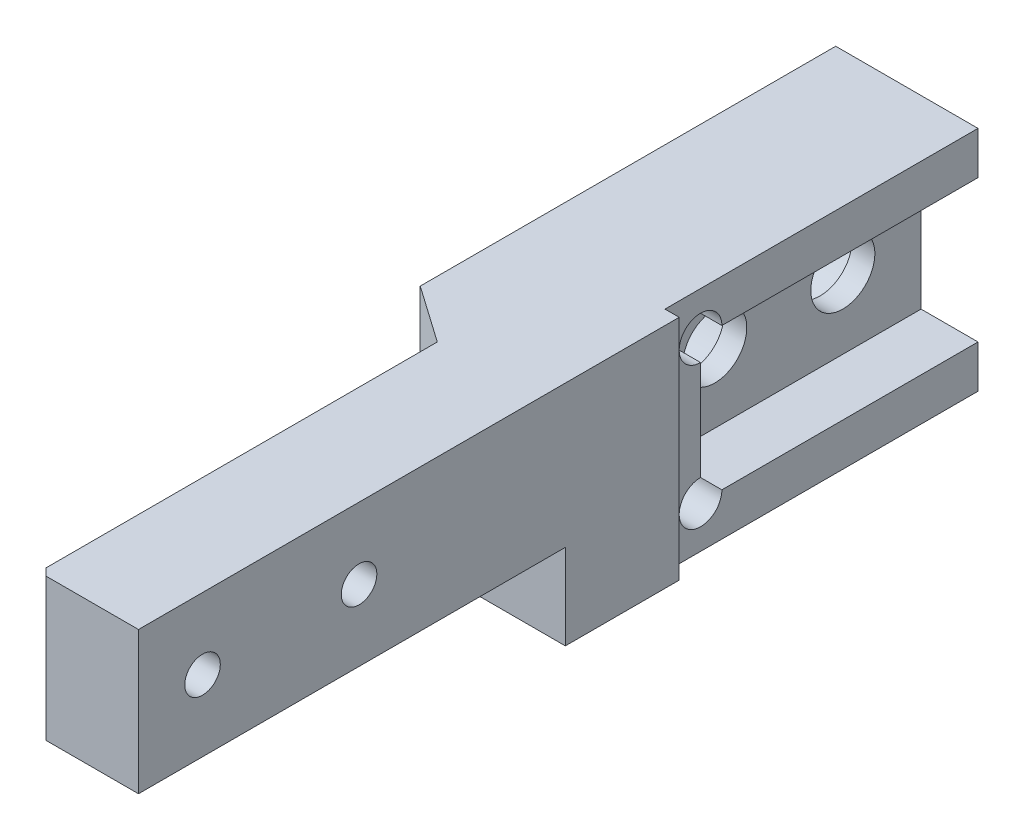
from build123d import *

# Parameters (mm, degrees)
SKETCH_1_W                   = 20
SKETCH_1_H                   = 60
EXTRUDE_1_DEPTH              = 8
SKETCH_2_W                   = 19.5
SKETCH_2_H                   = 10
CUT_EXTRUDE_1_DEPTH          = 14
CHAMFER_1_SIZE               = 3
CUT_EXTRUDE_3_DEPTH          = 36.440090293
CUT_EXTRUDE_3_DEPTH_BACK     = 36.440090293
CHAMFER_2_SIZE               = 0.5
SKETCH_6_R                   = 1.5
CUT_EXTRUDE_4_DEPTH          = 14
HOLE_WIZARD_M4_1_D           = 4.5
HOLE_WIZARD_M4_1_CBORE_D     = 8
HOLE_WIZARD_M4_1_CBORE_DEPTH = 4.4
SKETCH_11_W                  = 10
SKETCH_11_H                  = 22
CUT_EXTRUDE_7_DEPTH          = 36.440090293
SKETCH_12_W                  = 30
SKETCH_12_H                  = 6
CUT_EXTRUDE_8_DEPTH          = 37.932370625
CUT_EXTRUDE_9_DEPTH          = 34.166247904
FILLET_2_R                   = 3
SKETCH_14_W                  = 18.511605667
SKETCH_14_H                  = 56.283608206
CUT_EXTRUDE_10_DEPTH         = 36.440090293
HOLE_WIZARD_M3_1_D           = 2.5


with BuildPart() as part:
    # 草图1 → 凸台-拉伸1 (new, symmetric)
    with BuildSketch(Plane(origin=(0, 0, 0), x_dir=(1, 0, 0), z_dir=(0, 1, 0))):
        Rectangle(SKETCH_1_W, SKETCH_1_H)
    extrude(amount=EXTRUDE_1_DEPTH, both=True)

    # 草图2 → 切除-拉伸1 (cut)
    with BuildSketch(Plane(origin=(10, 0, 0), x_dir=(0, 0, -1), z_dir=(1, 0, 0))):
        with Locations((20.25, 0)):
            Rectangle(SKETCH_2_W, SKETCH_2_H)
    extrude(amount=-CUT_EXTRUDE_1_DEPTH, mode=Mode.SUBTRACT)

    # 倒角1
    chamfer_1_edges = [part.edges().sort_by_distance(p)[0] for p in [
        (10, -6.5, -30),
        (10, 6.5, -30),
    ]]
    chamfer(chamfer_1_edges, length=CHAMFER_1_SIZE)

    # 草图5 → 切除-拉伸3 (cut, two sides: drawn at the far end of the back side and taken through both)
    with BuildSketch(Plane.XZ.offset(8).offset(-CUT_EXTRUDE_3_DEPTH_BACK)):
        Polygon((-6, 164.19339757), (-6, 30), (-6, 2), (-10, -0.800830153), (-119.92479595, -77.771000913), (-362.743295595, 36.555933952), (-248.818499645, 278.520332435), align=None)
    extrude(amount=CUT_EXTRUDE_3_DEPTH + CUT_EXTRUDE_3_DEPTH_BACK, mode=Mode.SUBTRACT)

    # 倒角2
    chamfer_2_edges = [part.edges().sort_by_distance(p)[0] for p in [
        (-6, 0, 30),
        (10, 0, 30),
    ]]
    chamfer(chamfer_2_edges, length=CHAMFER_2_SIZE)

    # 草图6 → 切除-拉伸4 (cut)
    with BuildSketch(Plane(origin=(10, 0, 0), x_dir=(0, 0, -1), z_dir=(1, 0, 0))):
        with Locations((10.5, 5)):
            Circle(SKETCH_6_R)
        with Locations((10.5, -5)):
            Circle(SKETCH_6_R)
    extrude(amount=-CUT_EXTRUDE_4_DEPTH, mode=Mode.SUBTRACT)

    # M4 六角凹头螺钉的柱形沉头孔1 (through all)
    with Locations(Plane.ZY.offset(10)):
        with Locations((-15.500000304, 6.53e-07), (-24.500000304, 6.53e-07)):
            CounterBoreHole(HOLE_WIZARD_M4_1_D / 2, HOLE_WIZARD_M4_1_CBORE_D / 2, HOLE_WIZARD_M4_1_CBORE_DEPTH)

    # 草图11 → 切除-拉伸7 (cut, through all)
    with BuildSketch(Plane.XZ.offset(8)):
        with Locations((5, -19)):
            Rectangle(SKETCH_11_W, SKETCH_11_H)
    extrude(amount=-CUT_EXTRUDE_7_DEPTH, mode=Mode.SUBTRACT)

    # 草图12 → 切除-拉伸8 (cut, through all)
    with BuildSketch(Plane(origin=(10, 0, 0), x_dir=(0, 0, -1), z_dir=(1, 0, 0))):
        with Locations((-15, -5)):
            Rectangle(SKETCH_12_W, SKETCH_12_H)
    extrude(amount=-CUT_EXTRUDE_8_DEPTH, mode=Mode.SUBTRACT)

    # 草图13 → 切除-拉伸9 (cut, through all)
    with BuildSketch(Plane.XZ.offset(2)):
        Polygon((10, 14.214190818), (5.948732796, 20), (10, 25.785809182), align=None)
    extrude(amount=-CUT_EXTRUDE_9_DEPTH, mode=Mode.SUBTRACT)

    # 圆角2
    fillet_2_edges = [part.edges().sort_by_distance(p)[0] for p in [
        (5.948732796, 3, 20),
    ]]
    fillet(fillet_2_edges, radius=FILLET_2_R)

    # 草图14 → 切除-拉伸10 (cut, through all)
    with BuildSketch(Plane(origin=(0, 8, 0), x_dir=(1, 0, 0), z_dir=(0, 1, 0))):
        with Locations((10.255802834, -12.692083527)):
            Rectangle(SKETCH_14_W, SKETCH_14_H)
    extrude(amount=-CUT_EXTRUDE_10_DEPTH, mode=Mode.SUBTRACT)

    # M3 螺纹孔1 (through all)
    with Locations(Plane(origin=(1, 0, 0), x_dir=(0, 0, -1), z_dir=(1, 0, 0))):
        with Locations((-25.5, 3), (-14.5, 3)):
            Hole(HOLE_WIZARD_M3_1_D / 2)


solid = part.part
